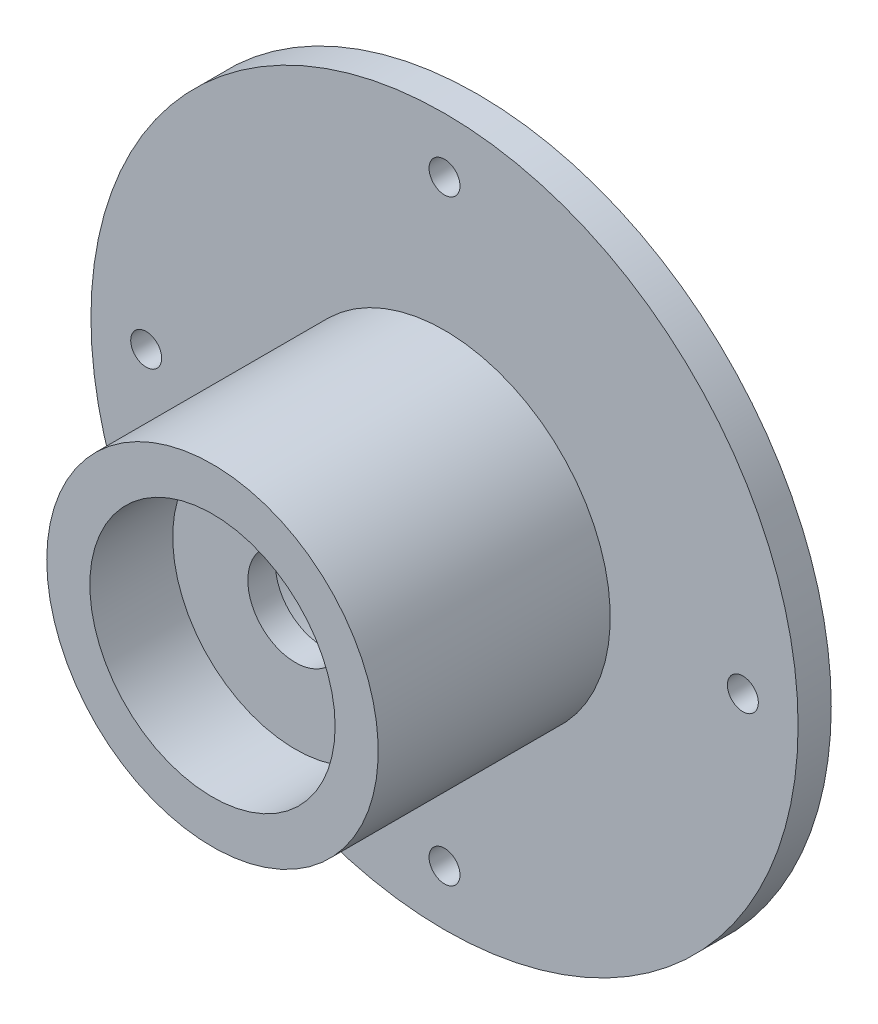
from build123d import *

# Parameters (mm, degrees)
SKETCH1_W                  = 32
SKETCH1_H                  = 3
SKETCH2_R                  = 15
BOSS_EXTRUDE1_DEPTH        = 21
F_2_8_2_8_DIAMETER_HOLE1_D = 2.8


with BuildPart() as part:
    # Sketch1 → Revolve1 (revolve)
    with BuildSketch(Plane(origin=(0, 0, 0), x_dir=(1, 0, 0), z_dir=(0, 1, 0))):
        with Locations((16, -1.5)):
            Rectangle(SKETCH1_W, SKETCH1_H)
    revolve(axis=Axis((0, 0, 0), (0, 0, 1)))

    # Sketch2 → Boss-Extrude1 (add)
    with BuildSketch(Plane.XY.offset(3)):
        with Locations(Location((0, 0, 0), (0, 0, 180))):
            Circle(SKETCH2_R)
    extrude(amount=BOSS_EXTRUDE1_DEPTH)

    # Sketch3 → Cut-Revolve1 (revolve, cut)
    with BuildSketch(Plane(origin=(0, 0, 0), x_dir=(1, 0, 0), z_dir=(0, 1, 0))):
        Polygon((13, 0), (0, 0), (0, -24), (11.1, -24), (11.1, -16.5), (4.3, -16.5), (4.3, -14), (13, -14), align=None)
    revolve(axis=Axis((0, 0, 0), (0, 0, 1)), mode=Mode.SUBTRACT)

    # Ø2.8 (2.8) Diameter Hole1 (through all)
    with Locations(Plane.XY.offset(3)):
        with Locations((0, 27), (0, -27), (27, 0), (-27, 0)):
            Hole(F_2_8_2_8_DIAMETER_HOLE1_D / 2)


solid = part.part
